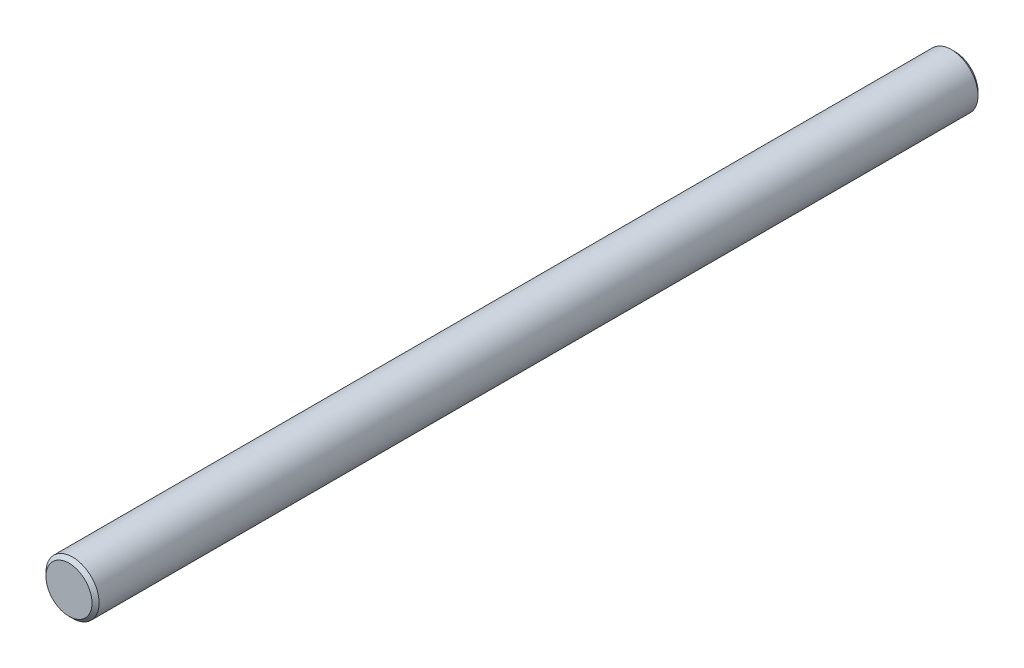
SolidWorks part; units mm, degrees
ref_plane "Front Plane" through (0, 0, 0) normal (0, 0, 1) x (1, 0, 0)
ref_plane "Top Plane" through (0, 0, 0) normal (0, 1, 0) x (1, 0, 0)
ref_plane "Right Plane" through (0, 0, 0) normal (1, 0, 0) x (0, 0, -1)
sketch "Sketch1" plane through (0, 0, 0) normal (0, 0, 1) x (1, 0, 0)
  circle A0 centre (0, 0) radius 1.5
  dimension "D1" = 3
extrude "Boss-Extrude1" add sketch "Sketch1" along normal blind 50
sketch "Sketch2" plane through (0, 0, 0) normal (0, 1, 0) x (1, 0, 0)
  line L0 (-1.5, 0) -> (-1.5, -50) construction
  line L1 (-1.5, -2) -> (-1, -2)
  line L2 (-1.5, -2) -> (-1.5, -6)
  line L3 (-1.5, -6) -> (-1, -6)
  line L4 (-1, -2) -> (-1, -6)
  line L5 (1.5, 0) -> (-1.5, 0) construction
  dimension "D1" = 0.5
  dimension "D2" = 2
  dimension "D3" = 4
extrude "Cut-Extrude1" cut sketch "Sketch2" against normal mid plane 30
chamfer "Chamfer1" distance 0.2 angle 45 2 edges at (1.5, 0, 50) (1.5, 0, 0)
